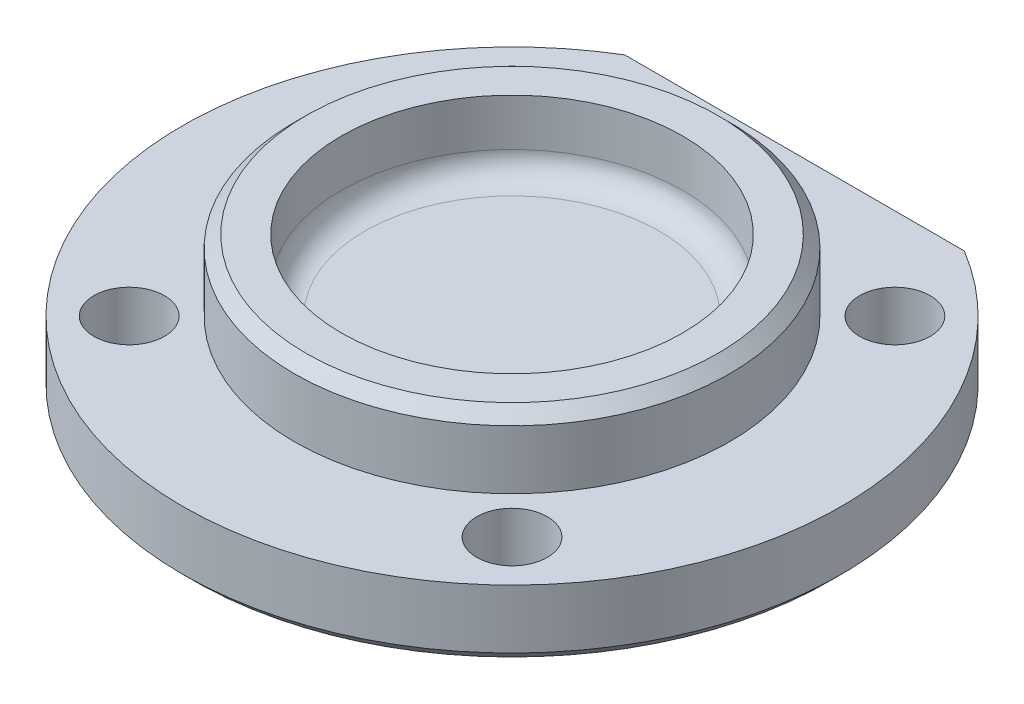
from build123d import *

# Parameters (mm, degrees)
SKETCH1_R           = 28
BOSS_EXTRUDE1_DEPTH = 6
SKETCH2_R           = 18.5
BOSS_EXTRUDE2_DEPTH = 6
SKETCH3_R           = 14.5
CUT_EXTRUDE1_DEPTH  = 6
FILLET2_R           = 2
CHAMFER1_SIZE       = 1
SKETCH4_R           = 3
CUT_EXTRUDE2_DEPTH  = 6
SKETCH5_W           = 48.146036261
SKETCH5_H           = 7.706921361
CUT_EXTRUDE3_DEPTH  = 6


with BuildPart() as part:
    # Sketch1 → Boss-Extrude1 (new body)
    with BuildSketch(Plane(origin=(0, 0, 0), x_dir=(1, 0, 0), z_dir=(0, 1, 0))):
        with Locations(Location((0, 0, 0), (0, 0, 270))):
            Circle(SKETCH1_R)
    extrude(amount=BOSS_EXTRUDE1_DEPTH)

    # Sketch2 → Boss-Extrude2 (add)
    with BuildSketch(Plane(origin=(0, 6, 0), x_dir=(1, 0, 0), z_dir=(0, 1, 0))):
        with Locations(Location((0, 0, 0), (0, 0, 270))):
            Circle(SKETCH2_R)
    extrude(amount=BOSS_EXTRUDE2_DEPTH)

    # Sketch3 → Cut-Extrude1 (cut)
    with BuildSketch(Plane(origin=(0, 12, 0), x_dir=(1, 0, 0), z_dir=(0, 1, 0))):
        with Locations(Location((0, 0, 0), (0, 0, 270))):
            Circle(SKETCH3_R)
    extrude(amount=-CUT_EXTRUDE1_DEPTH, mode=Mode.SUBTRACT)

    # Fillet2
    fillet2_edges = [part.edges().sort_by_distance(p)[0] for p in [
        (0, 6, -14.5),
    ]]
    fillet(fillet2_edges, radius=FILLET2_R)

    # Chamfer1
    chamfer1_edges = [part.edges().sort_by_distance(p)[0] for p in [
        (0, 0, -28),
        (0, 12, -18.5),
    ]]
    chamfer(chamfer1_edges, length=CHAMFER1_SIZE)

    # Sketch4 → Cut-Extrude2 (cut)
    with BuildSketch(Plane(origin=(0, 6, 0), x_dir=(1, 0, 0), z_dir=(0, 1, 0))):
        with Locations(Location((-16.263455967, 16.263455967, 0), (0, 0, 270))):
            Circle(SKETCH4_R)
        with Locations(Location((16.263455967, 16.263455967, 0), (0, 0, 270))):
            Circle(SKETCH4_R)
        with Locations(Location((16.263455967, -16.263455967, 0), (0, 0, 270))):
            Circle(SKETCH4_R)
        with Locations(Location((-16.263455967, -16.263455967, 0), (0, 0, 270))):
            Circle(SKETCH4_R)
    extrude(amount=-CUT_EXTRUDE2_DEPTH, mode=Mode.SUBTRACT)

    # Sketch5 → Cut-Extrude3 (cut)
    with BuildSketch(Plane(origin=(0, 6, 0), x_dir=(1, 0, 0), z_dir=(0, 1, 0))):
        with Locations((2.860896385, 27.85346068)):
            Rectangle(SKETCH5_W, SKETCH5_H)
    extrude(amount=-CUT_EXTRUDE3_DEPTH, mode=Mode.SUBTRACT)


solid = part.part
